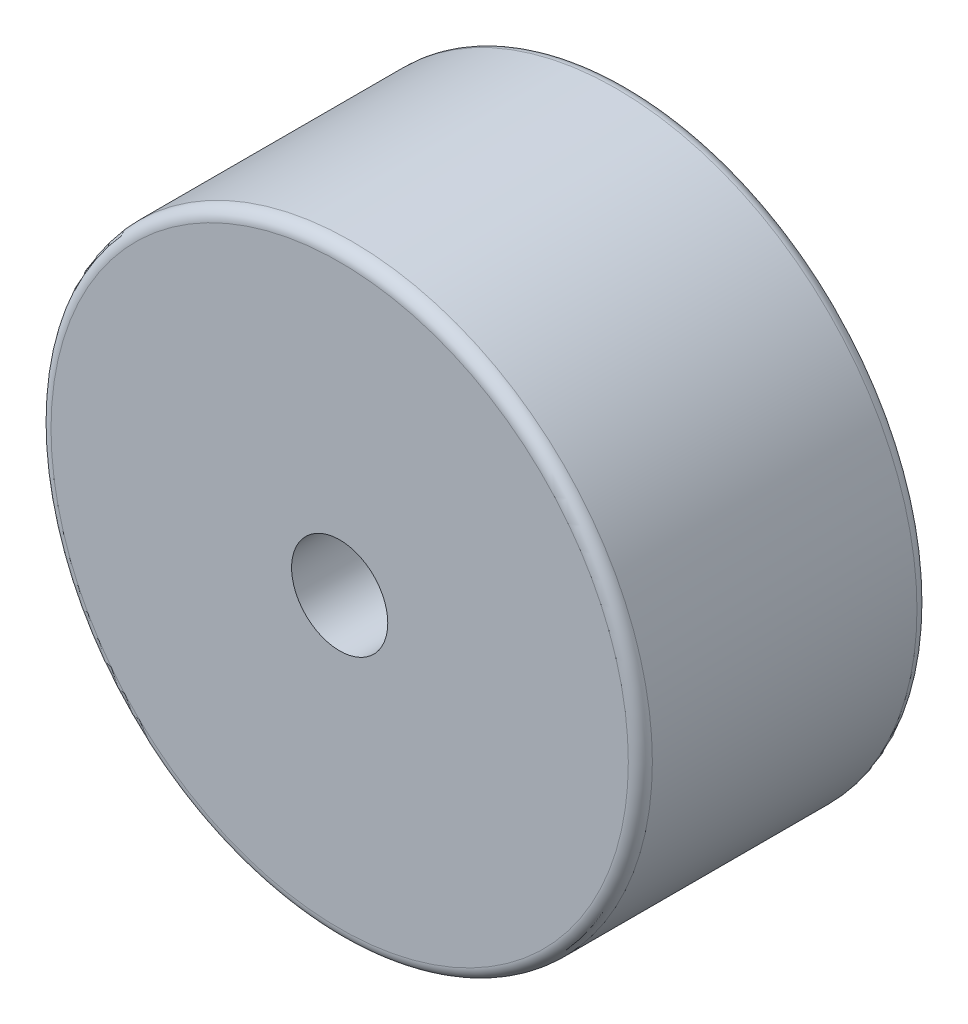
SolidWorks part; units mm, degrees
ref_plane "前视基准面" through (0, 0, 0) normal (0, 0, 1) x (1, 0, 0)
ref_plane "上视基准面" through (0, 0, 0) normal (0, 1, 0) x (1, 0, 0)
ref_plane "右视基准面" through (0, 0, 0) normal (1, 0, 0) x (0, 0, -1)
sketch "草图1" plane through (0, 0, 0) normal (0, 0, 1) x (1, 0, 0)
  circle A0 centre (0, 0) radius 25
  dimension "D1" = 50
extrude "凸台-拉伸1" add sketch "草图1" along normal blind 24
sketch "草图2" plane through (0, 0, 24) normal (0, 0, 1) x (1, 0, 0)
  circle A0 centre (0, 0) radius 4
  dimension "D1" = 8
extrude "切除-拉伸1" cut sketch "草图2" against normal blind 24
fillet "圆角1" radius 1 2 edges at (25, 0, 0) (25, 0, 24)
